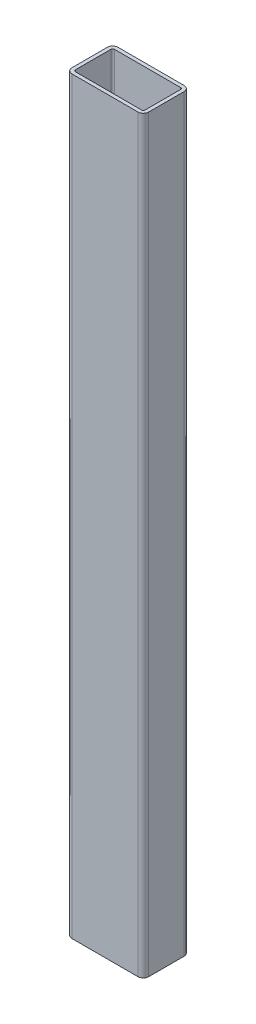
SolidWorks part; units mm, degrees
ref_plane "Front" through (0, 0, 0) normal (0, 0, 1) x (1, 0, 0)
ref_plane "Top" through (0, 0, 0) normal (0, 1, 0) x (1, 0, 0)
ref_plane "Right" through (0, 0, 0) normal (1, 0, 0) x (0, 0, -1)
sketch "Sketch1" plane through (0, 0, 0) normal (0, 1, 0) x (1, 0, 0)
  line L0 (-21.55, -12.7) -> (21.55, -12.7)
  line L1 (-21.55, -15) -> (21.55, -15)
  line L2 (-25, -11.55) -> (-25, 11.55)
  line L3 (-21.55, 15) -> (21.55, 15)
  line L4 (25, -11.55) -> (25, 11.55)
  line L5 (-25, -15) -> (25, 15) construction
  line L6 (-25, 15) -> (25, -15) construction
  line L7 (22.7, -11.55) -> (22.7, 11.55)
  line L8 (-21.55, 12.7) -> (21.55, 12.7)
  line L9 (-22.7, -11.55) -> (-22.7, 11.55)
  arc A0 (21.55, 15) -> (25, 11.55) centre (21.55, 11.55) cw
  arc A1 (-21.55, -15) -> (-25, -11.55) centre (-21.55, -11.55) cw
  arc A2 (21.55, -15) -> (25, -11.55) centre (21.55, -11.55) ccw
  arc A3 (-25, 11.55) -> (-21.55, 15) centre (-21.55, 11.55) cw
  arc A4 (21.55, -12.7) -> (22.7, -11.55) centre (21.55, -11.55) ccw
  arc A5 (21.55, 12.7) -> (22.7, 11.55) centre (21.55, 11.55) cw
  arc A6 (-22.7, 11.55) -> (-21.55, 12.7) centre (-21.55, 11.55) cw
  arc A7 (-21.55, -12.7) -> (-22.7, -11.55) centre (-21.55, -11.55) cw
  point P0 (0, 0)
  dimension "D3" = 3.45
  dimension "D1" = 50
  dimension "D2" = 30
  dimension "D4" = 2.3
extrude "Boss-Extrude1" add sketch "Sketch1" along normal blind 488
